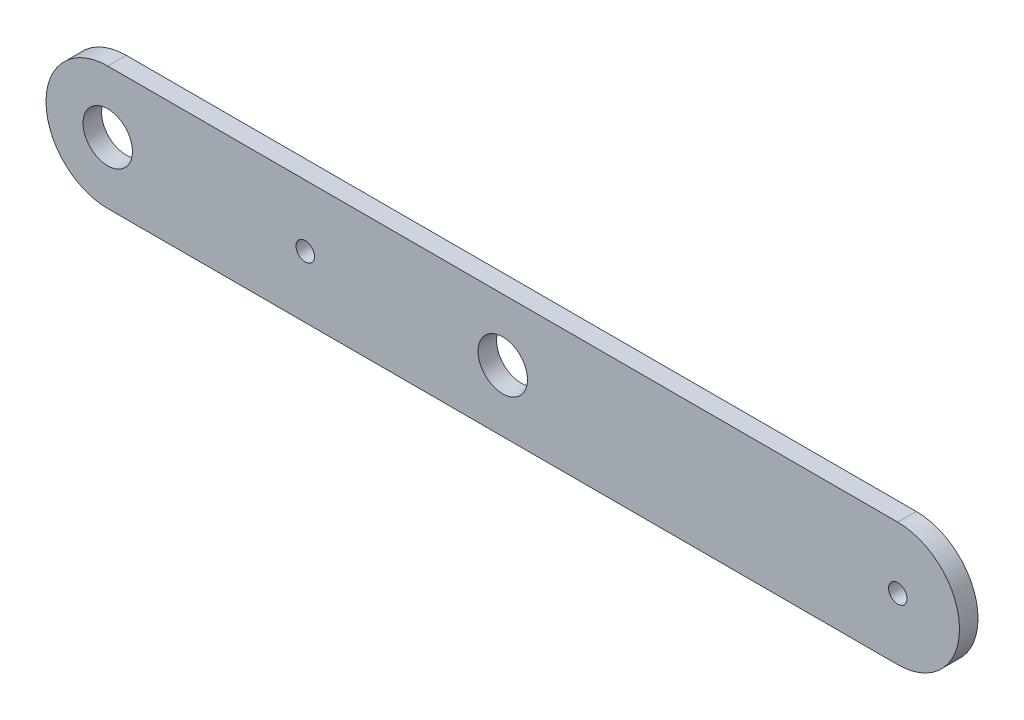
SolidWorks part; units mm, degrees
ref_plane "Front plane" through (0, 0, 0) normal (0, 0, 1) x (1, 0, 0)
ref_plane "Top plane" through (0, 0, 0) normal (0, 1, 0) x (1, 0, 0)
ref_plane "Right plane" through (0, 0, 0) normal (1, 0, 0) x (0, 0, -1)
sketch "Sketch 1" plane through (0, 0, 0) normal (0, 0, 1) x (1, 0, 0)
  line L0 (-57.2993, 0) -> (6.7007, 0) construction
  line L1 (-57.2993, 5) -> (6.7007, 5)
  line L2 (-57.2993, -5) -> (6.7007, -5)
  arc A0 (-57.2993, 5) -> (-57.2993, -5) centre (-57.2993, 0) ccw
  arc A1 (6.7007, -5) -> (6.7007, 5) centre (6.7007, 0) ccw
  circle A2 centre (-57.2993, 0) radius 2
  circle A3 centre (6.7007, 0) radius 0.75
  circle A4 centre (-41.2993, 0) radius 0.75
  circle A5 centre (-25.2993, 0) radius 2
  point P3 (-25.2993, 0)
  dimension "D2" = 5
  dimension "D4" = 4
  dimension "D5" = 4
  dimension "D6" = 1.5
  dimension "D8" = 1.5
  dimension "D1" = 48
  dimension "D3" = 16
  dimension "D7" = 16
extrude "Boss-Extrude 1" add sketch "Sketch 1" along normal blind 1.5
